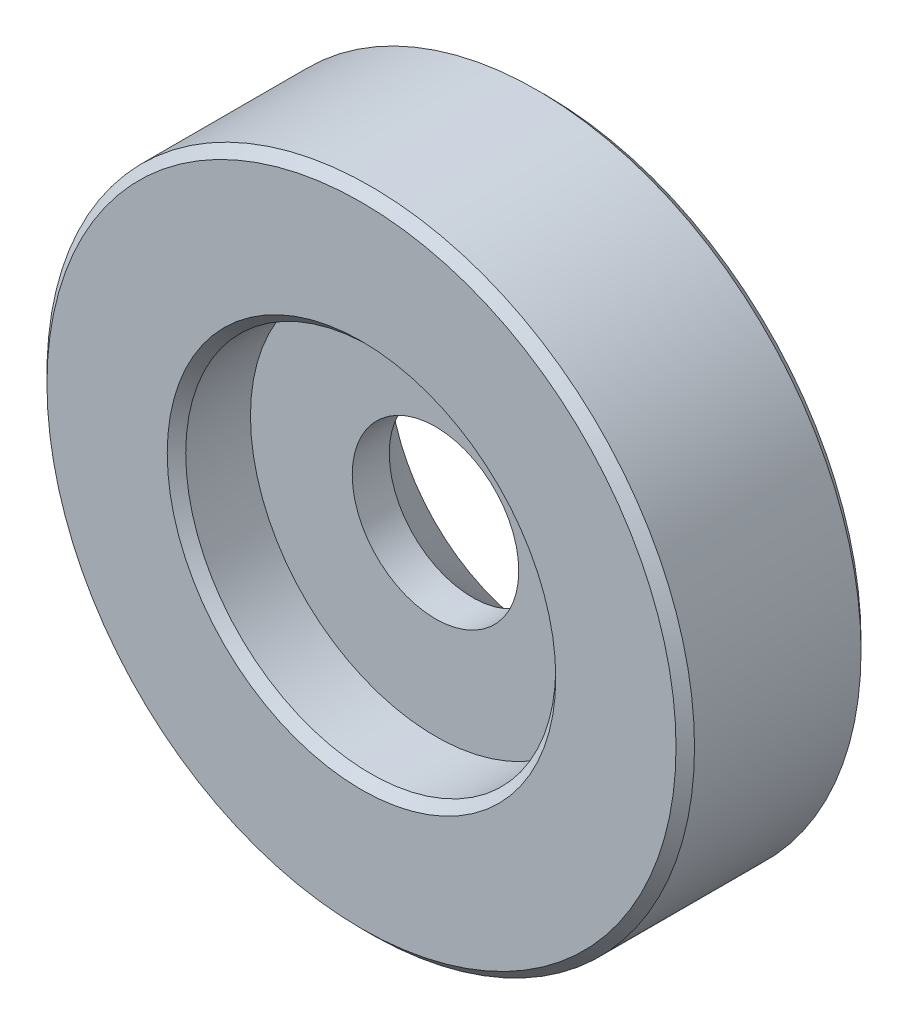
SolidWorks part; units mm, degrees
material "P20"
ref_plane "Front Plane" through (0, 0, 0) normal (0, 0, 1) x (1, 0, 0)
ref_plane "Top Plane" through (0, 0, 0) normal (0, 1, 0) x (1, 0, 0)
ref_plane "Right Plane" through (0, 0, 0) normal (1, 0, 0) x (0, 0, -1)
sketch "Sketch1" plane through (0, 0, 0) normal (0, 0, 1) x (1, 0, 0)
  circle A1 centre (0, 0) radius 17.5
  dimension "D2" = 35
extrude "Boss-Extrude1" add sketch "Sketch1" along normal blind 10
chamfer "Chamfer1" distance 0.5 angle 45 2 edges at (17.5, 0, 10) (17.5, 0, 0)
hole_wizard "Hole size (per socket flat counteBLZKk head screw type)1" positions "Sketch3" profile "Sketch2" countersink size "M8" standard "GB" end condition through all
sketch "Sketch3" plane through (0, 0, 0) normal (0, 0, 1) x (1, 0, 0)
  point P0 (0, 0)
  dimension "D1" = 0
sketch "Sketch2" plane through (0, 0, 0) normal (1, 0, 0) x (0, 1, 0)
  line L0 (0, 0) -> (0, 10)
  line L1 (0, 10) -> (4.5, 10)
  line L2 (4.5, 10) -> (4.5, 4)
  line L3 (4.5, 4) -> (8.5, 0)
  line L5 (8.5, 0) -> (0, 0)
  line L6 (-4.5, 4) -> (-8.5, 0) construction
  line L11 (0, -6.35) -> (0, 107.95) construction
  dimension "通孔孔直径" = 9
  dimension "通孔孔深度" = 10
  dimension "近端锥形沉头孔直径" = 17
  dimension "近端锥形沉头孔角度" = 90
sketch "Sketch5" plane through (0, 0, 10) normal (0, 0, 1) x (1, 0, 0)
  circle A0 centre (0, 0) radius 10
  dimension "D1" = 20
extrude "Cut-Extrude1" cut sketch "Sketch5" against normal blind 4
chamfer "Chamfer2" distance 0.5 angle 45 1 edges at (10, 0, 10)
